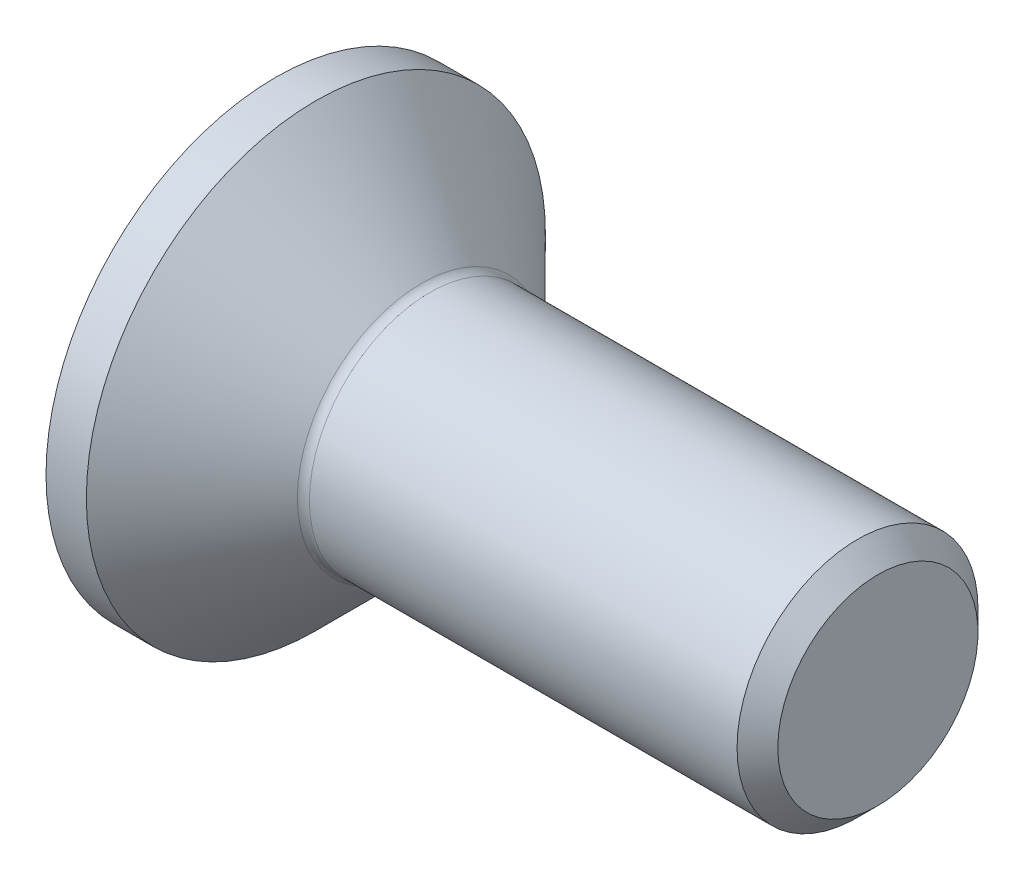
from build123d import *

# Parameters (mm, degrees)
HEXAGONSOCKET_DEPTH = 3
HEADFILLET_R        = 0.4
CHAMFER_2_SIZE      = 0.6765
SKETCH4_W           = 5
SKETCH4_H           = 5


with BuildPart() as part:
    # Sketch1 → Base (revolve)
    with BuildSketch(Plane.XY, mode=Mode.PRIVATE) as base_sk:
        Polygon((0, 0), (0, 8.96), (4.96, 4), (20, 4), (20, 0), align=None)
    revolve(base_sk.sketch.rotate(Axis((-0.587069181, 0, 0), (1, 0, 0)), 90), axis=Axis((-0.587069181, 0, 0), (1, 0, 0)))

    # Sketch2 → HexagonSocket (cut)
    with BuildSketch(Plane(origin=(0, 0, 0), x_dir=(0, 0, -1), z_dir=(1, 0, 0))):
        Polygon((2.886751346, 0), (1.443375673, 2.5), (-1.443375673, 2.5), (-2.886751346, 0), (-1.443375673, -2.5), (1.443375673, -2.5), align=None)
    extrude(amount=HEXAGONSOCKET_DEPTH, mode=Mode.SUBTRACT)

    # Sketch3 → Cut-Revolve1 (revolve, cut)
    with BuildSketch(Plane.XY, mode=Mode.PRIVATE) as cut_revolve1_sk:
        Polygon((3, 2.5), (4.443375673, 0), (3, 0), align=None)
    revolve(cut_revolve1_sk.sketch.rotate(Axis((-0.439109555, 0, 0), (1, 0, 0)), 90), axis=Axis((-0.439109555, 0, 0), (1, 0, 0)), mode=Mode.SUBTRACT)

    # HeadFillet
    headfillet_edges = [part.edges().sort_by_distance(p)[0] for p in [
        (4.96, 0, -4),
    ]]
    fillet(headfillet_edges, radius=HEADFILLET_R)

    # Chamfer 2
    chamfer_2_edges = [part.edges().sort_by_distance(p)[0] for p in [
        (20, 0, -4),
    ]]
    chamfer(chamfer_2_edges, length=CHAMFER_2_SIZE)

    # Sketch4 → Cut-Revolve2 (revolve, cut)
    with BuildSketch(Plane(origin=(0, 0, 0), x_dir=(1, 0, 0), z_dir=(0, 1, 0)), mode=Mode.PRIVATE) as cut_revolve2_sk:
        with Locations((0.5, 10.12)):
            Rectangle(SKETCH4_W, SKETCH4_H)
    revolve(cut_revolve2_sk.sketch.rotate(Axis((11.853138686, 0, 0), (-1, 0, 0)), 180), axis=Axis((11.853138686, 0, 0), (-1, 0, 0)), mode=Mode.SUBTRACT)


solid = part.part
